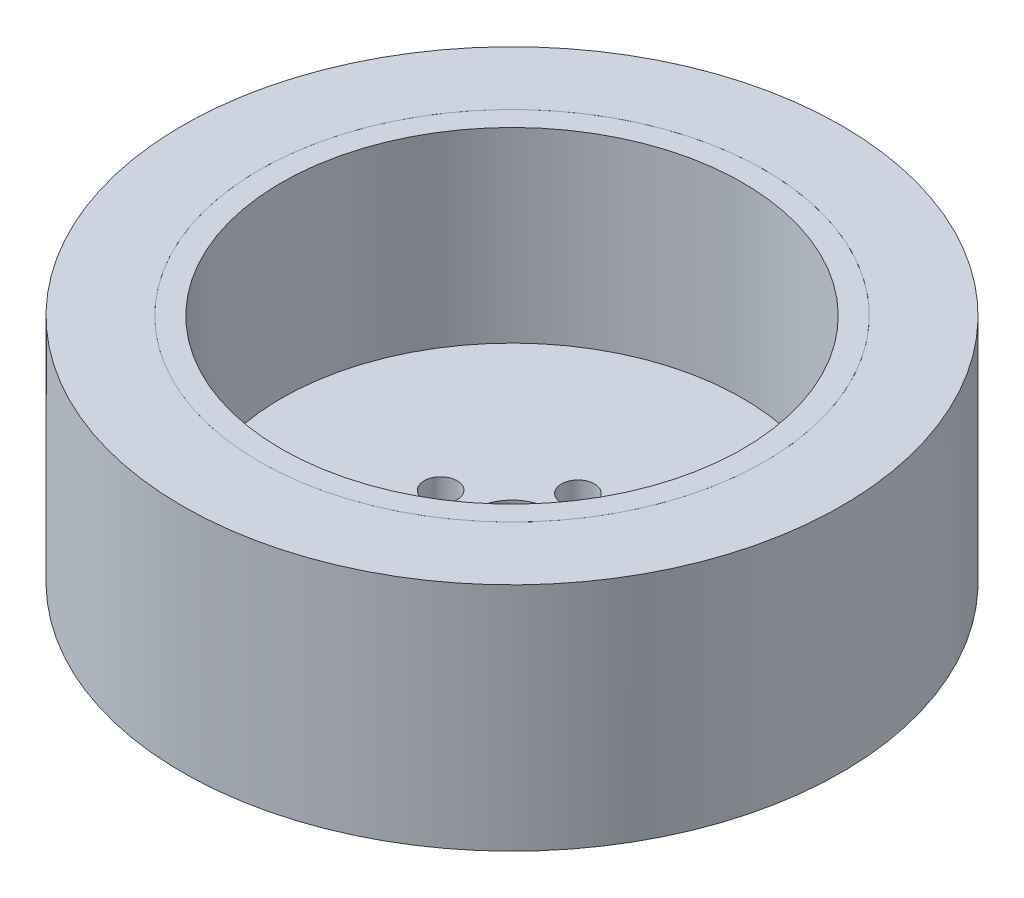
SolidWorks part; units mm, degrees
other "轮毂"
other "包胶"
ref_plane "Front Plane" through (0, 0, 0) normal (0, 0, 1) x (1, 0, 0)
ref_plane "Top Plane" through (0, 0, 0) normal (0, 1, 0) x (1, 0, 0)
ref_plane "Right Plane" through (0, 0, 0) normal (1, 0, 0) x (0, 0, -1)
sketch "Hub body definition" plane through (0, 0, 0) normal (0, 1, 0) x (1, 0, 0)
  line L0 (-6.5, 0) -> (6.5, 0) construction
  line L1 (0, 6) -> (0, -6) construction
  circle A0 centre (0, 0) radius 23
  circle A1 centre (0, 0) radius 3.5
  circle A2 centre (0, 0) radius 21 construction
  circle A3 centre (0, 6) radius 1.5
  circle A4 centre (0, -6) radius 1.5
  circle A5 centre (-6.5, 0) radius 1.5
  circle A6 centre (6.5, 0) radius 1.5
  dimension "D1" = 46
  dimension "D2" = 42
  dimension "D3" = 12
  dimension "D5" = 3
  dimension "D6" = 7
  dimension "D4" = 13
sketch "Sketch1" plane through (0, 0, 0) normal (0, 1, 0) x (1, 0, 0)
  circle A9 centre (6.5, 0) radius 1.5
  circle A10 centre (6.5, 0) radius 1.5
  circle A11 centre (-6.5, 0) radius 1.5
  circle A12 centre (-6.5, 0) radius 1.5
  circle A13 centre (0, -6) radius 1.5
  circle A14 centre (0, -6) radius 1.5
  circle A15 centre (0, 6) radius 1.5
  circle A16 centre (0, 6) radius 1.5
  circle A17 centre (0, 0) radius 3.5
  circle A18 centre (0, 0) radius 3.5
  circle A19 centre (0, 0) radius 23
  circle A20 centre (0, 0) radius 23
  dimension "D1" = 0
  dimension "D3" = 0
  dimension "D4" = 0
  dimension "D5" = 0
  dimension "D6" = 0
  dimension "D2" = 0
extrude "Boss-Extrude1" add sketch "Sketch1" along normal blind 4
sketch "Sketch2" plane through (0, 4, 0) normal (0, 1, 0) x (1, 0, 0)
  circle A0 centre (0, 0) radius 21 construction
  circle A1 centre (0, 0) radius 21
  circle A15 centre (0, 0) radius 23
  circle A16 centre (0, 0) radius 23
  dimension "D6" = 0
extrude "Boss-Extrude2" add sketch "Sketch2" along normal blind 17
sketch "Sketch3" plane through (0, 0, 0) normal (0, -1, 0) x (1, 0, 0)
  circle A2 centre (0, 0) radius 30
  circle A14 centre (0, 0) radius 23
  circle A15 centre (0, 0) radius 23
  dimension "D1" = 60
  dimension "D7" = 0
extrude "Boss-Extrude3" add sketch "Sketch3" against normal up to surface (21 mm away) separate body up to face at (0, 21, 23)
